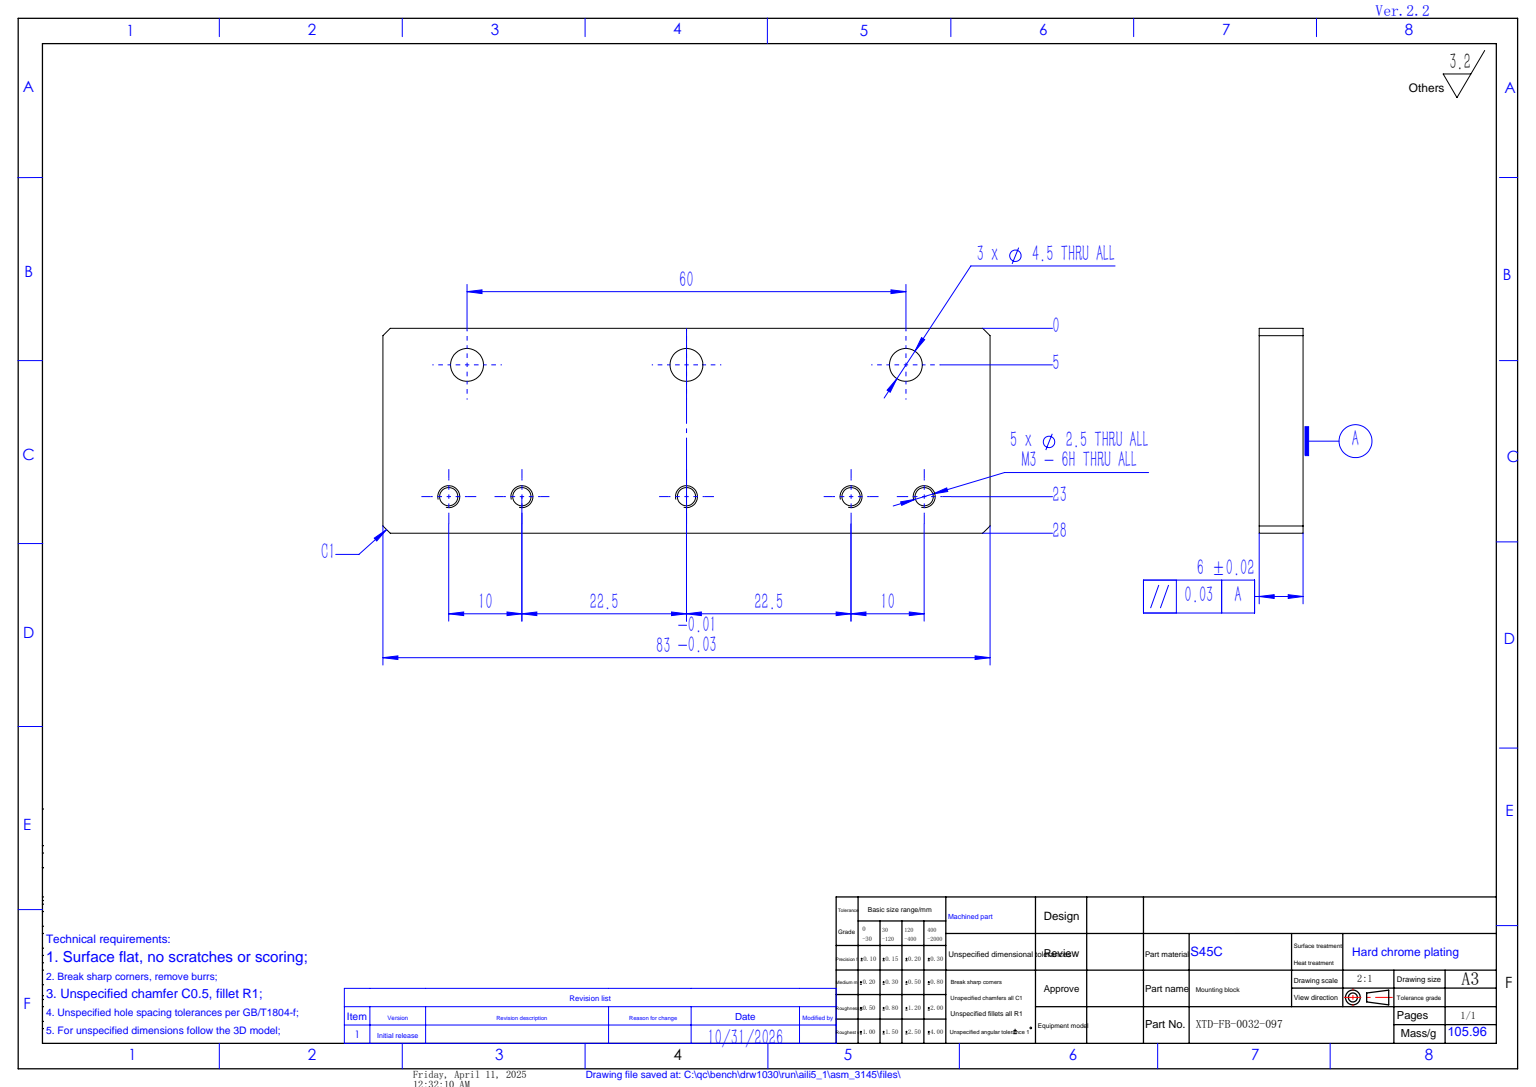
from build123d import *

# Parameters (mm, degrees)
SKETCH_1_W         = 83
SKETCH_1_H         = 28
EXTRUDE_1_DEPTH    = 6
HOLE_WIZARD_M4_1_D = 4.5
HOLE_WIZARD_M3_1_D = 2.5
CHAMFER_1_SIZE     = 1


with BuildPart() as part:
    # 草图1 → 凸台-拉伸1 (new body)
    with BuildSketch(Plane.XY):
        Rectangle(SKETCH_1_W, SKETCH_1_H)
    extrude(amount=EXTRUDE_1_DEPTH)

    # M4 间隙孔1 (through all)
    with Locations(Plane.XY.offset(6)):
        with Locations((-30, 9), (0, 9), (30, 9)):
            Hole(HOLE_WIZARD_M4_1_D / 2)

    # M3 螺纹孔1 (through all)
    with Locations(Plane.XY.offset(6)):
        with Locations((-32.5, -9), (0, -9), (32.5, -9), (22.5, -9), (-22.5, -9)):
            Hole(HOLE_WIZARD_M3_1_D / 2)

    # 倒角1
    chamfer_1_edges = [part.edges().sort_by_distance(p)[0] for p in [
        (41.5, -14, 3),
        (-41.5, -14, 3),
        (-41.5, 14, 3),
        (41.5, 14, 3),
    ]]
    chamfer(chamfer_1_edges, length=CHAMFER_1_SIZE)


solid = part.part
